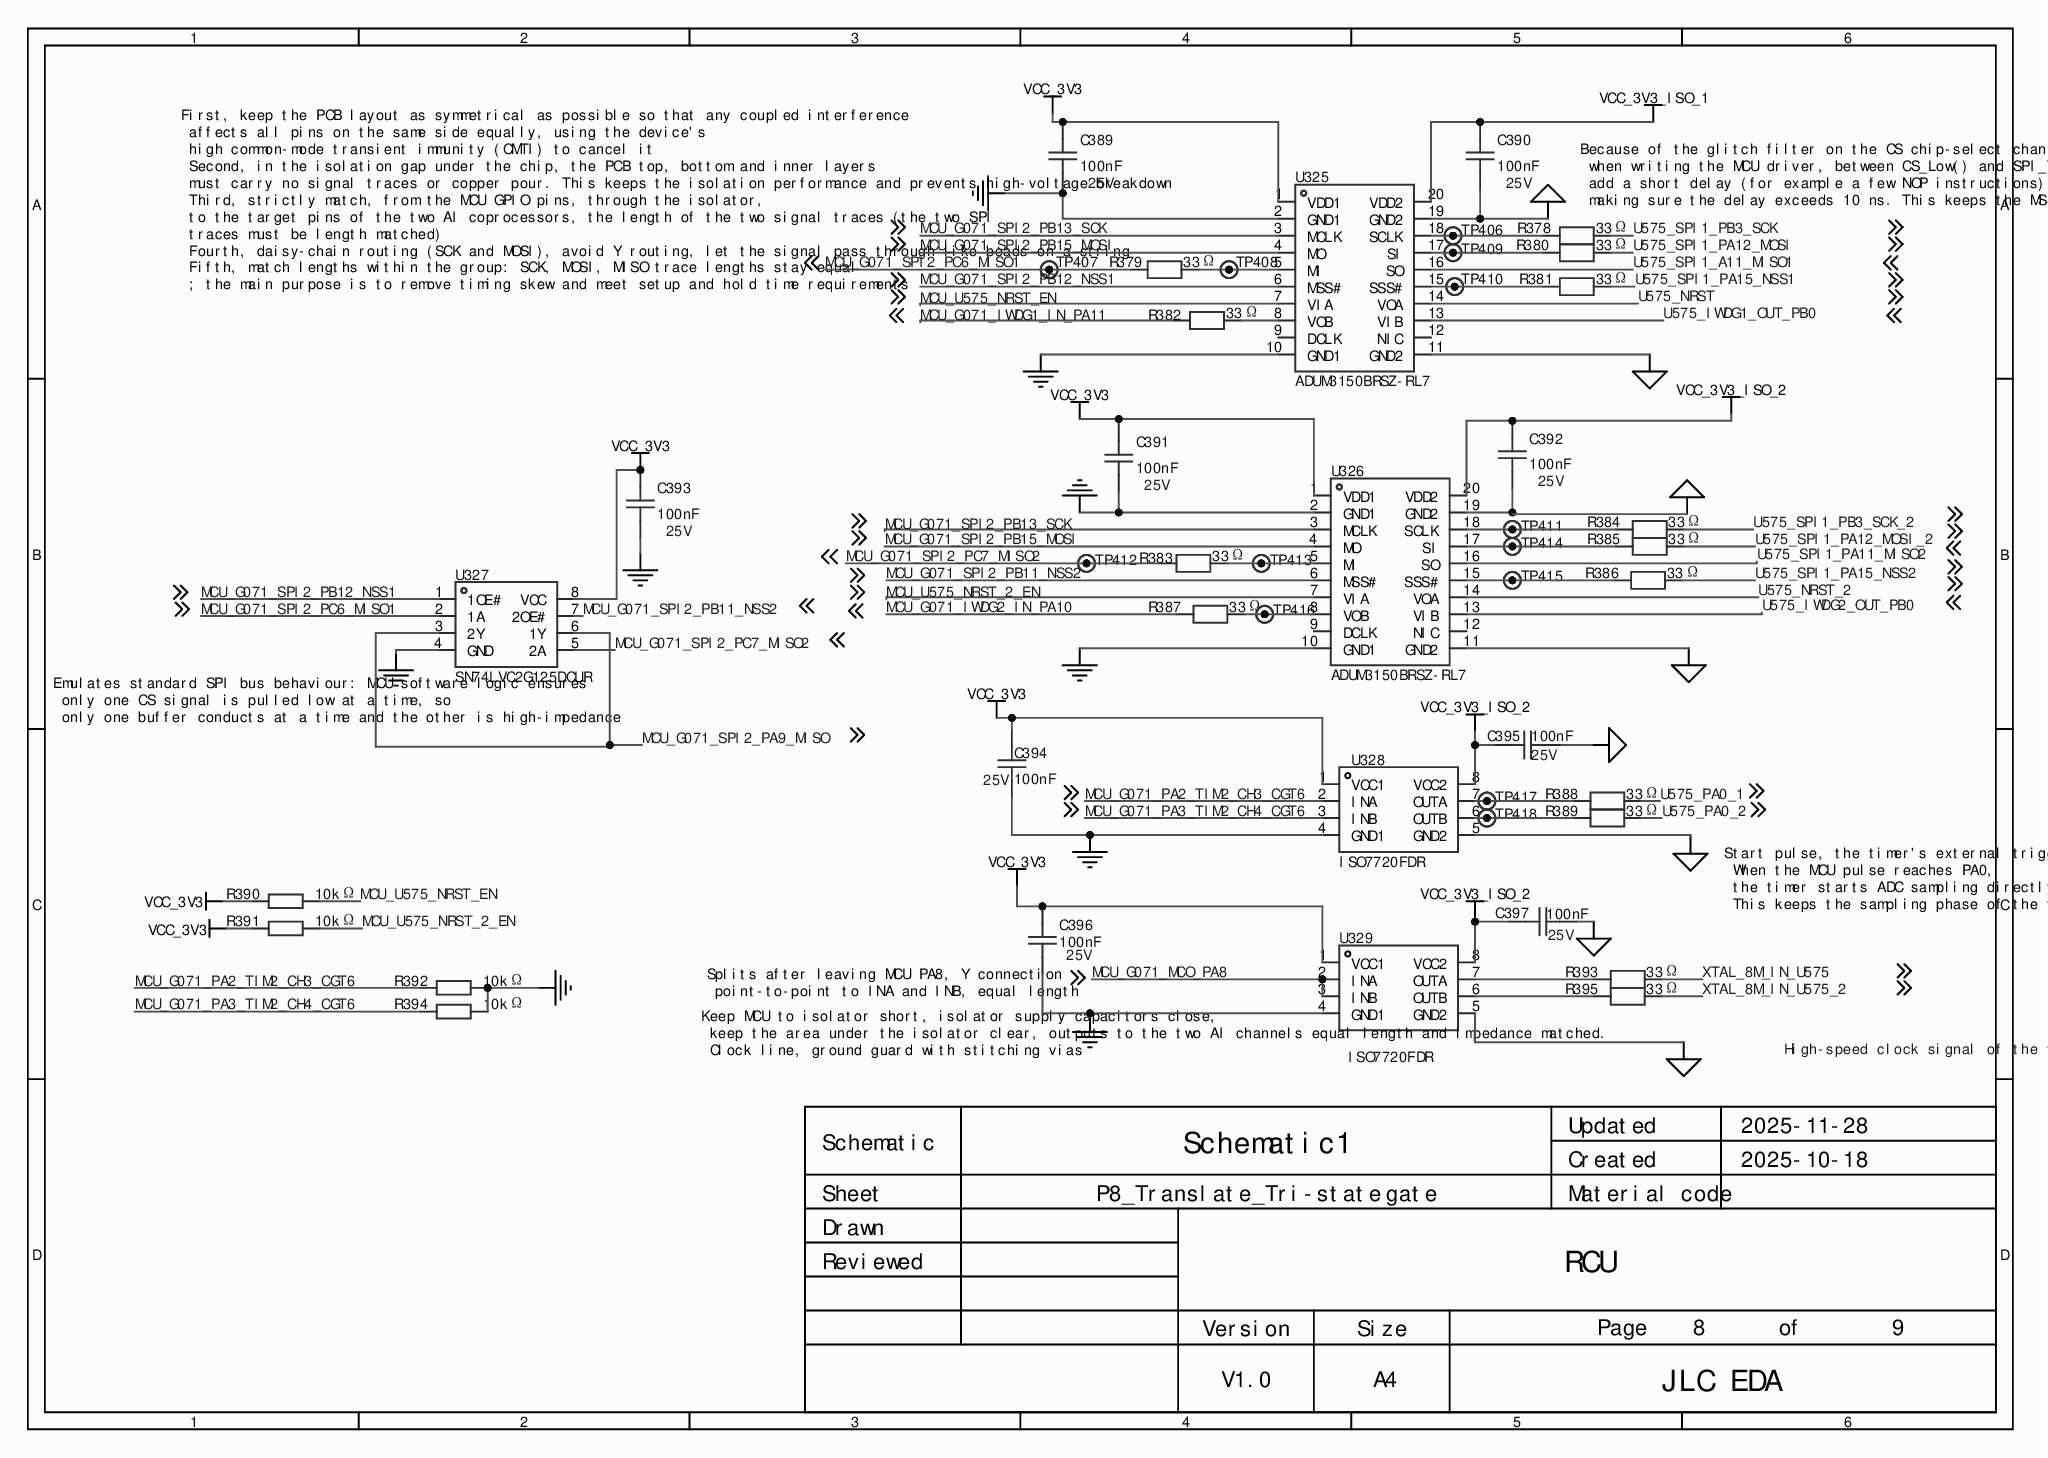
[diagram p0: MISC84429-10.SchDoc]
# Altium project MISC84429-12.PrjPcb (part 5 of 5)
## Sheet MISC84429-10.SchDoc (continued)
### Nets (continued)
U575_PA0_1: R388.1
U575_PA0_2: R389.1
U575_SPI1_A11_MISO1: U325.16(SO)
U575_SPI1_PA11_MISO2: U326.16(SO)
U575_SPI1_PA12_MOSI: R380.1
U575_SPI1_PA12_MOSI_2: R385.1
U575_SPI1_PA15_NSS1: R381.1
U575_SPI1_PA15_NSS2: R386.1
U575_SPI1_PB3_SCK: R378.1
U575_SPI1_PB3_SCK_2: R384.1
XTAL_8M_IN_U575: R393.1
XTAL_8M_IN_U575_2: R395.1
NetR378_2: R378.2 TP406.1 U325.18(SCLK)
NetR379_1: R379.1 TP408.1 U325.5(MI)
NetR380_2: R380.2 TP409.1 U325.17(SI)
NetR381_2: R381.2 TP410.1 U325.15(SSS#)
NetR382_1: R382.1 U325.8(VOB)
NetR383_1: R383.1 TP413.1 U326.5(MI)
NetR384_2: R384.2 TP411.1 U326.18(SCLK)
NetR385_2: R385.2 TP414.1 U326.17(SI)
NetR386_2: R386.2 TP415.1 U326.15(SSS#)
NetR387_1: R387.1 TP416.1 U326.8(VOB)
NetR388_2: R388.2 TP417.1 U328.7(OUTA)
NetR389_2: R389.2 TP418.1 U328.6(OUTB)
NetR393_2: R393.2 U329.7(OUTA)
NetR395_2: R395.2 U329.6(OUTB)

Not connected (* = marked no-connect by the designer): U325 9(DCLK)* 12(NIC)*; U326 9(DCLK)* 12(NIC)*

### Notes on the sheet
- First, keep the PCB layout as symmetrical as possible so that any coupled interference
  affects all pins on the same side equally, using the device's
  high common-mode transient immunity (CMTI) to cancel it
  Second, in the isolation gap under the chip, the PCB top, bottom and inner layers
  must carry no signal traces or copper pour. This keeps the isolation performance and prevents high-voltage breakdown
  Third, strictly match, from the MCU GPIO pins, through the isolator,
  to the target pins of the two AI coprocessors, the length of the two signal traces (the two SPI
  traces must be length matched)
  Fourth, daisy-chain routing (SCK and MOSI), avoid Y routing, let the signal pass through like beads on a string
  Fifth, match lengths within the group: SCK, MOSI, MISO trace lengths stay equal
  ; the main purpose is to remove timing skew and meet setup and hold time requirements
- Because of the glitch filter on the CS chip-select channel,
  when writing the MCU driver, between CS_Low() and SPI_Transmit()
  add a short delay (for example a few NOP instructions),
  making sure the delay exceeds 10 ns. This keeps the MSS setup time above 10ns
- Emulates standard SPI bus behaviour: MCU software logic ensures
  only one CS signal is pulled low at a time, so
  only one buffer conducts at a time and the other is high-impedance
- Start pulse, the timer's external trigger source.
  When the MCU pulse reaches PA0,
  the timer starts ADC sampling directly through the hardware link.
  This keeps the sampling phase of the two AI channels fully aligned
- Keep MCU to isolator short, isolator supply capacitors close,
  keep the area under the isolator clear, outputs to the two AI channels equal length and impedance matched.
  Clock line, ground guard with stitching vias
- Splits after leaving MCU PA8, Y connection
  point-to-point to INA and INB, equal length
- High-speed clock signal of the two AI coprocessors
- 1
- 2
- 3
- 4
- 5
- 6
- A
- B
- C
- Schematic
- Schematic1
- Created
- Updated
- 2025-11-28
- 2025-10-18
- D
- Reviewed
- Drawn
- Sheet
- P8_Translate_Tri-state gate
- Material code
- RCU
- Version
- Size
- Page
- 8
- of
- 9
- V1.0
- A4
- JLC EDA

### Library data of the parts
C389-C397 = GRM188R71E104KA01D: as C381-C384 on sheet MISC84429-8; Symbol: GRM188R71E104KA01D; Device: GRM188R71E104KA01D; LCSC Part Name: 100nF ±10% 25V; Supplier Part: C77050; Manufacturer Part: GRM188R71E104KA01D; Supplier Footprint: 0603; JLCPCB Part Class: Extended library; Datasheet: https://atta.szlcsc.com/upload/public/pdf/source/20170622/1498103881034.pdf; Supplier: LCSC; Convert to PCB: yes; Value: 100nF; Origin Footprint: C0603
R378-R389 R393 R395 = FRC0603F33R0TS: as R372 on sheet MISC84429-8; Symbol: FRC0603F33R0TS; Device: FRC0603F33R0TS; LCSC Part Name: 33Ω ±1% 100mW 厚膜电阻; Supplier Part: C2909394; Manufacturer Part: FRC0603F33R0TS; Supplier Footprint: 0603; JLCPCB Part Class: Extended library; Supplier: LCSC; Convert to PCB: yes; Type: Thick film resistor; Value: 33Ω; Operating Temperature: -55℃~+155℃; Origin Footprint: R0603
R390-R392 R394 = RC0603FR-0710KL: as R371 on sheet MISC84429-8; Symbol: RC0603FR-0710KL; Device: RC0603FR-0710KL; LCSC Part Name: 厚膜电阻 10kΩ ±1% 100mW; Supplier Part: C98220; Manufacturer Part: RC0603FR-0710KL; Supplier Footprint: 0603; JLCPCB Part Class: Extended library; Datasheet: https://atta.szlcsc.com/upload/public/pdf/source/20180927/C295883_E8D83085EA81BD7DE0B2B681138C15EE.pdf; Supplier: LCSC; Convert to PCB: yes; Type: Thick film resistor; Value: 10kΩ; Operating Temperature Range: -55℃~+155℃; Origin Footprint: R0603
TP406-TP418 = Test-Point: Add into BOM: yes; Symbol: Test-Point; Device: Test-Point; Convert to PCB: yes; Origin Footprint: Test-Point-0.5mm
U325 U326 = ADUM3150BRSZ-RL7: Manufacturer: ADI(亚德诺); Add into BOM: yes; Symbol: ADUM3150BRSZ-RL7; Device: ADUM3150BRSZ-RL7; LCSC Part Name: 用于SPI高速接口的3.75 kV专用隔离器（1/1辅助通道方向性）; Supplier Part: C660732; Manufacturer Part: ADUM3150BRSZ-RL7; Supplier Footprint: SSOP-20-208mil; JLCPCB Part Class: Extended library; Datasheet: https://atta.szlcsc.com/upload/public/pdf/source/20200914/C660732_9A8AE148C659C7DDC4EF09AB6B6BF7D1.pdf; Supplier: LCSC; Convert to PCB: yes; Origin Footprint: SSOP-20_L7.2-W5.3-P0.65-LS7.8-BL
U327 = SN74LVC2G125DCUR: Manufacturer: TI(德州仪器); Add into BOM: yes; output type: Tri-state; Voltage - Supply: 1.65V~5.5V; Number of Elements: 2; Current - Output Low(IOL): 32mA; Logic Family: 74LVC; Quiescent Current: 10uA; Propagation Delay: 4.3ns@3.3V,50pF; Symbol: SN74LVC2G125DCUR; Device: SN74LVC2G125DCUR; LCSC Part Name: 双路三态输出总线缓冲门; Supplier Part: C21404; Manufacturer Part: SN74LVC2G125DCUR; Supplier Footprint: VSSOP-8; JLCPCB Part Class: Extended library; Datasheet: https://www.ti.com/cn/lit/gpn/sn74lvc2g125; Supplier: LCSC; Convert to PCB: yes; Input type: -; Current - Output High(IOH): 32mA; Operating Temperature: -40℃~+85℃; Origin Footprint: VSON8_L2.0-W2.3-P0.50-LS3.1-BL
U328 U329 = ISO7720FDR: Manufacturer: TI(德州仪器); Add into BOM: yes; Number of Forward Channels: 2; Number of Reverse Channels: 0; Data Rate(Max): 100Mbps; Isolation Voltage(Vrms): 5000; CMTI(kV/us): 100kV/us; Voltage - Supply(VCCA): 2.25V~5.5V; Propagation Delay(tpd): 11ns; Symbol: ISO7720FDR; Device: ISO7720FDR; LCSC Part Name: ISO772x高速双通道增强型数字隔离器; Supplier Part: C2878308; Manufacturer Part: ISO7720FDR; Supplier Footprint: SOIC-8; JLCPCB Part Class: Extended library; Datasheet: https://www.ti.com/cn/lit/gpn/iso7721; Supplier: LCSC; Convert to PCB: yes; Default Output: -; Operating Temperature: -55℃~+125℃; Voltage - Supply(VCCB): 2.25V~5.5V; Origin Footprint: SOIC-8_L5.0-W4.0-P1.27-LS6.1-BL

## Sheet MISC84429-9.SchDoc
size 309 x 223 mm; Name: Sheet-Symbol; Symbol: Sheet-Symbol; Device: Sheet-Symbol
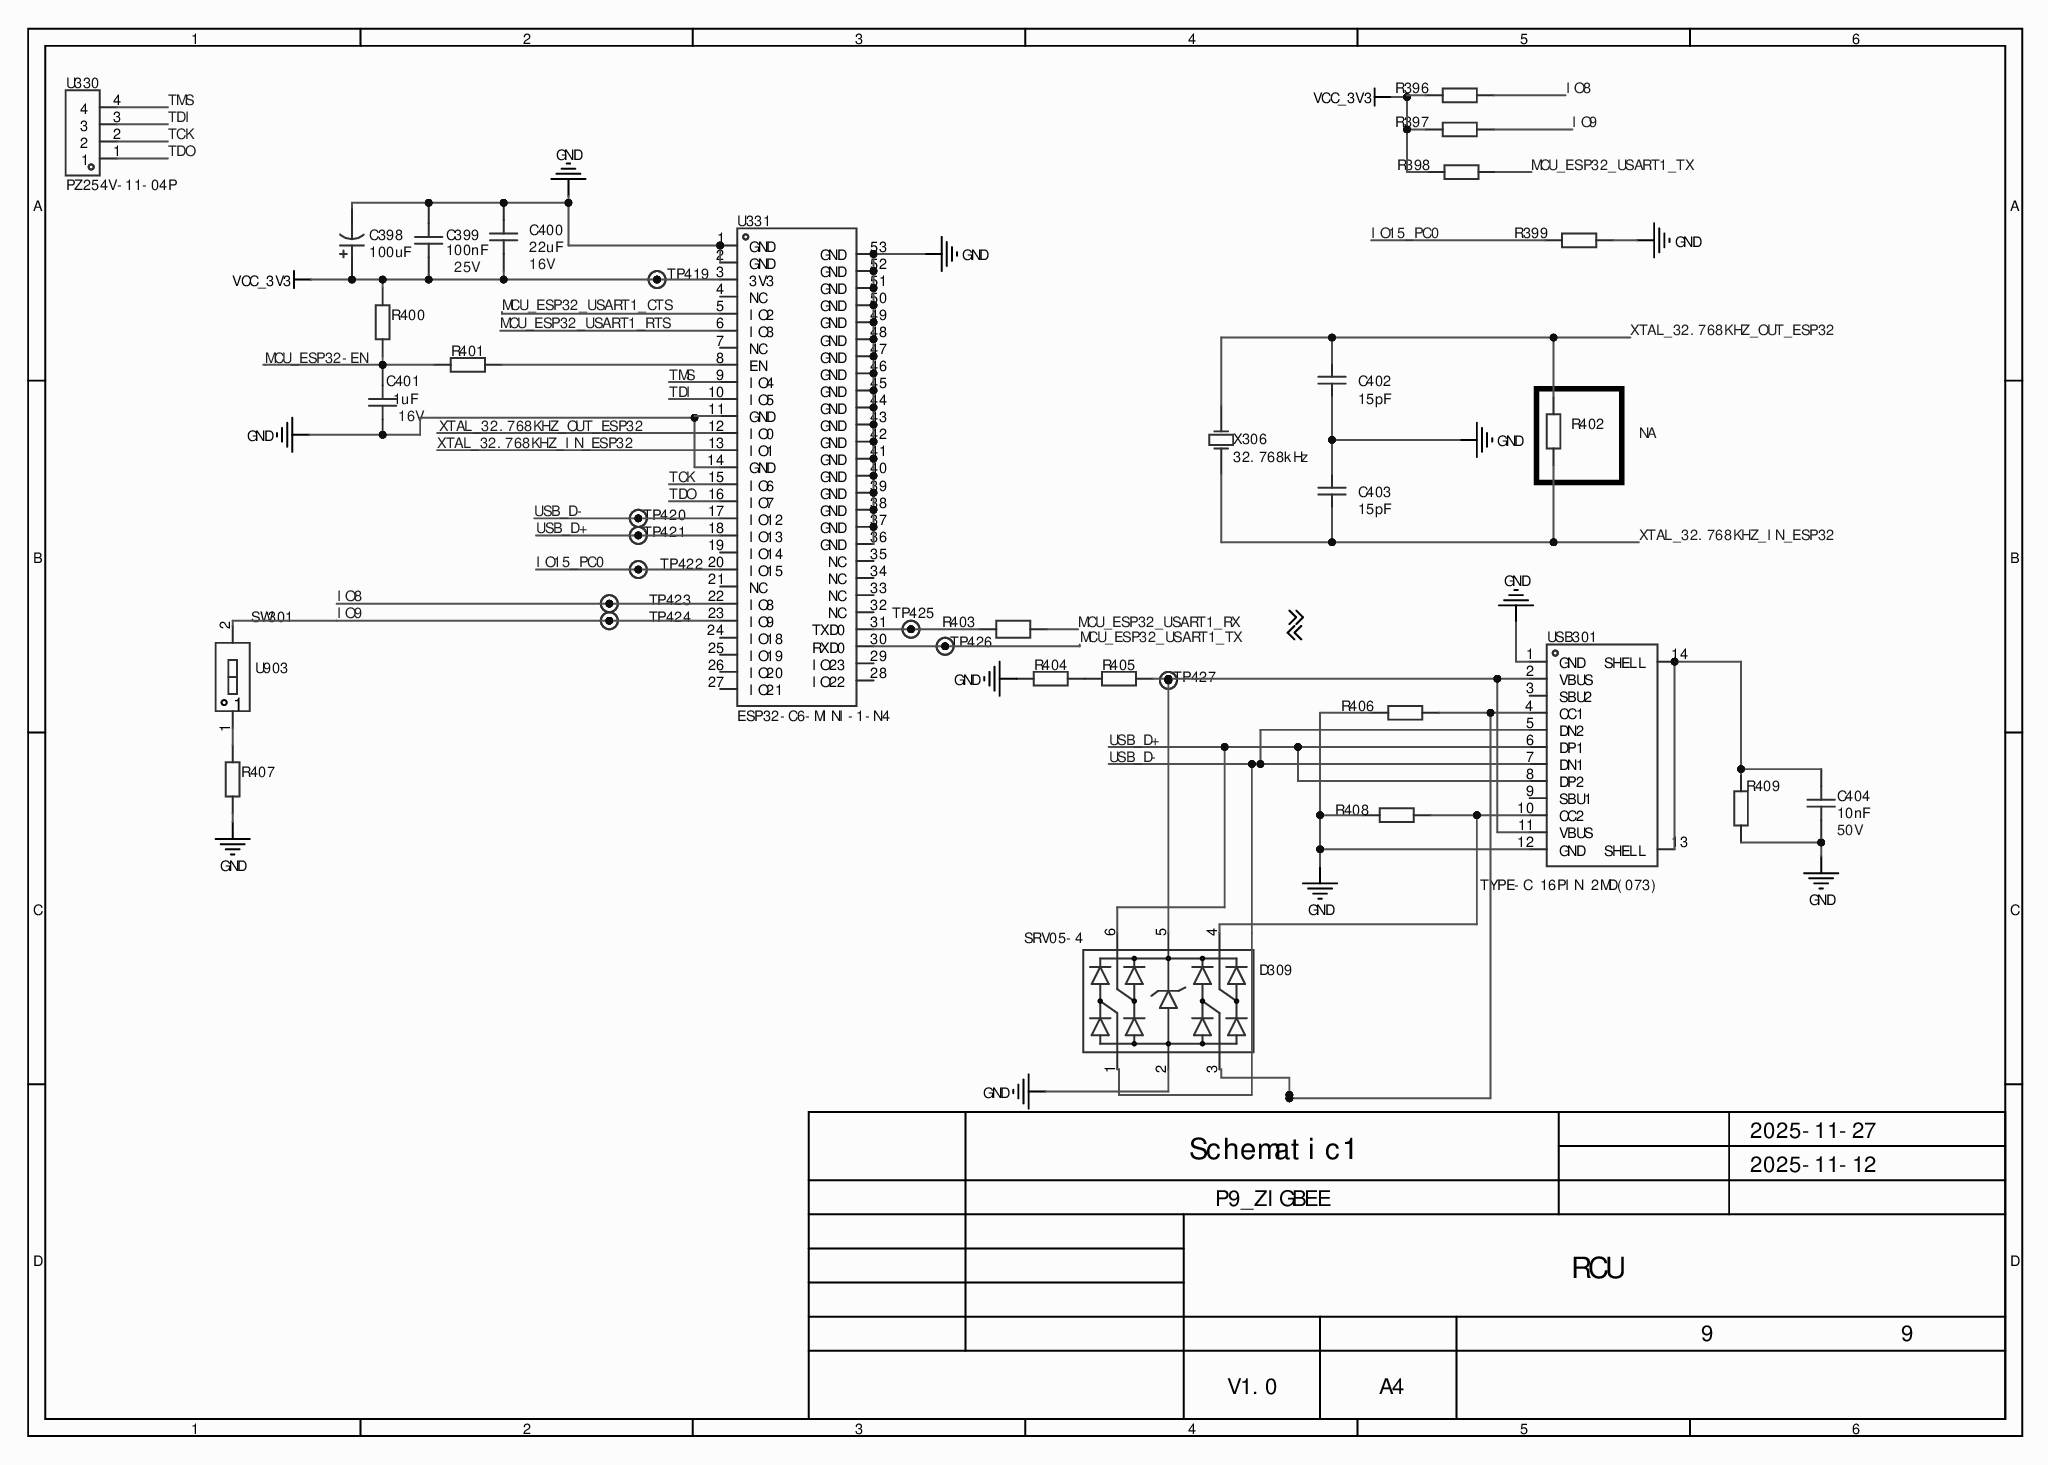
[diagram p1: MISC84429-9.SchDoc]

### Parts
C398  100uF  [CAP-SMD_BD6.3-L6.6-W6.6-LS7.2-FD]
C399  100nF  Voltage Rated: 25V  [C0603]
C400  22uF  Voltage Rating: 16V  [C0603]
C401  1uF  Voltage Rated: 16V  [C0603]
C402  15pF  [C0402]
C403  15pF  [C0402]
C404  10nF  Voltage Rating: 50V  [C0603]
D309  SRV05-4  [SOT-23-6_L2.9-W1.6-P0.95-LS2.8-BL]
R396  (no value)  [R0603]
R397  (no value)  [R0603]
R398  (no value)  [R0603]
R399  (no value)  [R0603]
R400  (no value)  [R0603]
R401  (no value)  [R0603]
R402  (no value)  [R0402]
R403  (no value)  [R0603]
R404  (no value)  [R0603]
R405  (no value)  [R0603]
R406  (no value)  [R0603]
R407  (no value)  [R0603]
R408  (no value)  [R0603]
R409  (no value)  [R0402]
SW301  U903  [SW-SMD_2P-L3.5-W6.1-P2.54-LS9.8]
TP419  (no value)  [Test-Point-0.5mm]
TP420  (no value)  [Test-Point-0.5mm]
TP421  (no value)  [Test-Point-0.5mm]
TP422  (no value)  [Test-Point-0.5mm]
TP423  (no value)  [Test-Point-0.5mm]
TP424  (no value)  [Test-Point-0.5mm]
TP425  (no value)  [Test-Point-0.5mm]
TP426  (no value)  [Test-Point-0.5mm]
TP427  (no value)  [Test-Point-0.5mm]
U330  PZ254V-11-04P  [HDR-TH_4P-P2.54-V-M]
U331  ESP32-C6-MINI-1-N4  [WIFIM-SMD_61P-L16.6-W13.2-P0.80-ESP32-C6-MINI-1-N4]
USB301  TYPE-C 16PIN 2MD(073)  [USB-C-SMD_TYPE-C-6PIN-2MD-073]
X306  32.768kHz  [OSC-TH_BD3.1-P0.8-D0.3]

### Nets
GND: C398.2 C399.1 C400.2 C401.1 C402.1 C403.2 C404.1 D309.2 R399.1 R404.2 R406.1 R407.1 R408.1 R409.1 U331.1(GND) U331.2(GND) U331.11(GND) U331.14(GND) U331.36(GND) U331.37(GND) U331.38(GND) U331.39(GND) U331.40(GND) U331.41(GND) U331.42(GND) U331.43(GND) U331.44(GND) U331.45(GND) U331.46(GND) U331.47(GND) U331.48(GND) U331.49(GND) U331.50(GND) U331.51(GND) U331.52(GND) U331.53(GND) USB301.1(GND) USB301.12(GND)
VCC_3V3: C398.1 C399.2 C400.1 R396.2 R397.2 R398.2 R400.2 TP419.1 U331.3(3V3)
IO8: R396.1 TP423.1 U331.22(IO8)
IO9: R397.1 SW301.2(PIN2) TP424.1 U331.23(IO9)
IO15_PC0: R399.2 TP422.1 U331.20(IO15)
MCU_ESP32-EN: C401.2 R400.1 R401.1
MCU_ESP32_USART1_CTS: U331.5(IO2)
MCU_ESP32_USART1_RTS: U331.6(IO3)
MCU_ESP32_USART1_RX: R403.1
MCU_ESP32_USART1_TX: R398.1 TP426.1 U331.30(RXD0)
TCK: U330.2 U331.15(IO6)
TDI: U330.3 U331.10(IO5)
TDO: U330.1 U331.16(IO7)
TMS: U330.4 U331.9(IO4)
USB_D+: D309.6 TP421.1 U331.18(IO13) USB301.6(DP1) USB301.8(DP2)
USB_D-: D309.1 TP420.1 U331.17(IO12) USB301.5(DN2) USB301.7(DN1)
XTAL_32.768KHZ_IN_ESP32: C403.1 R402.1 U331.13(IO1) X306.2(OSC2)
XTAL_32.768KHZ_OUT_ESP32: C402.2 R402.2 U331.12(IO0) X306.1(OSC1)
NetC404_2: C404.2 R409.2 USB301.13(SHELL) USB301.14(SHELL)
NetD309_3: D309.3 R406.2 USB301.4(CC1)
NetD309_4: D309.4 R408.2 USB301.10(CC2)
NetD309_5: D309.5 R405.2 TP427.1 USB301.2(VBUS) USB301.11(VBUS)
NetR401_2: R401.2 U331.8(EN)
NetR403_2: R403.2 TP425.1 U331.31(TXD0)
NetR404_1: R404.1 R405.1
NetR407_2: R407.2 SW301.1(PIN1)

Not connected (* = marked no-connect by the designer): U331 4(NC)* 7(NC)* 19(IO14)* 21(NC)* 24(IO18)* 25(IO19)* 26(IO20)* 27(IO21)* 28(IO22)* 29(IO23)* 32(NC)* 33(NC)* 34(NC)* 35(NC)*; USB301 3(SBU2)* 9(SBU1)*

### Notes on the sheet
- NA
- 1
- 2
- 3
- 4
- 5
- 6
- A
- B
- C
- Schematic1
- 2025-11-27
- 2025-11-12
- D
- P9_ZIGBEE
- RCU
- 9
- V1.0
- A4

### Library data of the parts
C398 = 100uF: Symbol: RVT100UF16V67RV0016; Add into BOM: yes; Voltage Rating: 16V; Ripple Current: 93mA@120Hz; Device: 100uF; Supplier Part: C2887276; Manufacturer Part: RVT100UF16V67RV0016; Supplier Footprint: SMD,D6.3xL5.4mm; Datasheet: https://atta.szlcsc.com/upload/public/pdf/source/20240521/3810EB5B434F72326C196D6A9426C70A.pdf; Supplier: LCSC; Convert to PCB: yes; Value: 100uF; Equivalent Series Resistance(ESR): -; Diameter: 6.3mm; Height - Seated (Max): 5.4mm; Origin Footprint: CAP-SMD_BD6.3-L6.6-W6.6-LS7.2-FD; Design Item ID: RVT100UF16V67RV0016
C399 = 100nF: Symbol: GRM188R71E104KA01D; Add into BOM: yes; Temperature Coefficient: X7R; Device: 100nF; Supplier Part: C77050; Manufacturer Part: GRM188R71E104KA01D; Supplier Footprint: 0603; Datasheet: https://atta.szlcsc.com/upload/public/pdf/source/20170622/1498103881034.pdf; Supplier: LCSC; Convert to PCB: yes; Value: 100nF; Origin Footprint: C0603; Design Item ID: GRM188R71E104KA01D
C400 = 22uF: Symbol: GRM188R61C226ME01D; Add into BOM: yes; Temperature Coefficient: X5R; Device: 22uF; Supplier Part: C5116073; Manufacturer Part: GRM188R61C226ME01D; Supplier Footprint: 0603; Datasheet: https://item.szlcsc.com/datasheet/GRM188R61C226ME01D/5691201.html; Supplier: LCSC; Convert to PCB: yes; Value: 22uF; Origin Footprint: C0603; Design Item ID: GRM188R61C226ME01D
C401 = 1uF: Symbol: GCM188R71C105KA64D; Add into BOM: yes; Temperature Coefficient: X7R; Device: 1uF; Supplier Part: C161212; Manufacturer Part: GCM188R71C105KA64D; Supplier Footprint: 0603; Datasheet: https://atta.szlcsc.com/upload/public/pdf/source/20181221/C161212_C96DD77354D5551432B3B7779E4D1948.pdf; Supplier: LCSC; Convert to PCB: yes; Value: 1uF; Origin Footprint: C0603; Design Item ID: GCM188R71C105KA64D
C402 C403 = 15pF: Symbol: GJM1555C1H150FB01D; Add into BOM: yes; Voltage Rated: 50V; Temperature Coefficient: C0G; Device: 15pF; Supplier Part: C441742; Manufacturer Part: GJM1555C1H150FB01D; Supplier Footprint: 0402; Datasheet: https://atta.szlcsc.com/upload/public/pdf/source/20200305/C490387_23319AE8C154DEB24C505E6C82A8106A.pdf; Supplier: LCSC; Convert to PCB: yes; Value: 15pF; Origin Footprint: C0402; Design Item ID: GJM1555C1H150FB01D
C404 = 10nF: Symbol: GCM188R71H103KA37D; Add into BOM: yes; Temperature Coefficient: X7R; Device: 10nF; Supplier Part: C85863; Manufacturer Part: GCM188R71H103KA37D; Supplier Footprint: 0603; Datasheet: https://item.szlcsc.com/datasheet/GCM188R71H103KA37D/87039.html; Supplier: LCSC; Convert to PCB: yes; Value: 10nF; Origin Footprint: C0603; Design Item ID: GCM188R71H103KA37D
D309 = SRV05-4: Symbol: SRV05-4_C558418; Add into BOM: yes; Reverse Stand-Off Voltage (Vrwm): 5V; Clamping Voltage: 20V; Peak Pulse Current (Ipp): 3A; Peak Pulse Power Dissipation (Ppp): 60W; Voltage - Breakdown: 6V; Reverse Leakage Current (Ir): 500nA; Type: ESD; Device: SRV05-4; Supplier Part: C558418; Manufacturer Part: SRV05-4; Supplier Footprint: SOT-23-6; Datasheet: https://item.szlcsc.com/datasheet/SRV05-4/581825.html; Supplier: LCSC; Convert to PCB: yes; Origin Footprint: SOT-23-6_L2.9-W1.6-P0.95-LS2.8-BL; Design Item ID: SRV05-4_C558418
R396-R399 R407 = RC0603FR-074K7L: Add into BOM: yes; Power(Watts): 100mW; Voltage-Supply(Max): 75V; Symbol: RC0603FR-074K7L; Device: RC0603FR-074K7L; Supplier Part: C99782; Manufacturer Part: RC0603FR-074K7L; Supplier Footprint: 0603; Datasheet: https://atta.szlcsc.com/upload/public/pdf/source/20250610/89E4D743C004A82A45145C7A2CC3A578.pdf; Supplier: LCSC; Convert to PCB: yes; Origin Footprint: R0603; Design Item ID: RC0603FR-074K7L
R400 R404 R405 = RC0603FR-0710KL: Add into BOM: yes; Power(Watts): 100mW; Overload Voltage (Max): 75V; Symbol: RC0603FR-0710KL; Device: RC0603FR-0710KL; Supplier Part: C98220; Manufacturer Part: RC0603FR-0710KL; Supplier Footprint: 0603; Datasheet: https://atta.szlcsc.com/upload/public/pdf/source/20180927/C295883_E8D83085EA81BD7DE0B2B681138C15EE.pdf; Supplier: LCSC; Convert to PCB: yes; Origin Footprint: R0603; Design Item ID: RC0603FR-0710KL
R401 = RC0603FR-070RL: Add into BOM: yes; Power(Watts): 100mW; Voltage-Supply(Max): 75V; Symbol: RC0603FR-070RL; Device: RC0603FR-070RL; Supplier Part: C100044; Manufacturer Part: RC0603FR-070RL; Supplier Footprint: 0603; Datasheet: https://item.szlcsc.com/datasheet/RC0603FR-070RL/101258.html; Supplier: LCSC; Convert to PCB: yes; Temperature Coefficient: -; Origin Footprint: R0603; Design Item ID: RC0603FR-070RL
R402 = 0402WGF1002TCE: Add into BOM: yes; Power(Watts): 62.5mW; Overload Voltage (Max): 50V; Symbol: 0402WGF1002TCE; Device: 0402WGF1002TCE; Supplier Part: C25744; Manufacturer Part: 0402WGF1002TCE; Supplier Footprint: 0402; Datasheet: https://atta.szlcsc.com/upload/public/pdf/source/20200306/C422600_1E6D84923E4A46A82E41ADD87F860B5C.pdf; Supplier: LCSC; Convert to PCB: yes; Origin Footprint: R0402; Design Item ID: 0402WGF1002TCE
R403 = FRC0603F33R0TS: Add into BOM: yes; Power(Watts): 100mW; Voltage-Supply(Max): 75V; Symbol: FRC0603F33R0TS; Device: FRC0603F33R0TS; Supplier Part: C2909394; Manufacturer Part: FRC0603F33R0TS; Supplier Footprint: 0603; Supplier: LCSC; Convert to PCB: yes; Origin Footprint: R0603; Design Item ID: FRC0603F33R0TS
R406 R408 = RC0603FR-075K1L: Add into BOM: yes; Power(Watts): 100mW; Voltage-Supply(Max): 75V; Symbol: RC0603FR-075K1L; Device: RC0603FR-075K1L; Supplier Part: C105580; Manufacturer Part: RC0603FR-075K1L; Supplier Footprint: 0603; Datasheet: https://atta.szlcsc.com/upload/public/pdf/source/20180316/70C0E2BDAE7FCC62C531A5A58D202EE1.pdf; Supplier: LCSC; Convert to PCB: yes; Origin Footprint: R0603; Design Item ID: RC0603FR-075K1L
R409 = 0402WGF1004TCE: Add into BOM: yes; Power(Watts): 62.5mW; Overload Voltage (Max): 50V; Symbol: 0402WGF1004TCE; Device: 0402WGF1004TCE; Supplier Part: C26083; Manufacturer Part: 0402WGF1004TCE; Supplier Footprint: 0402; Datasheet: https://atta.szlcsc.com/upload/public/pdf/source/20200306/C422600_1E6D84923E4A46A82E41ADD87F860B5C.pdf; Supplier: LCSC; Convert to PCB: yes; Origin Footprint: R0402; Design Item ID: 0402WGF1004TCE
SW301 = U903: Symbol: DSIC01LS-P; Add into BOM: yes; Current Rating: 25mA; Voltage Rating: 24V; Device: U903; Supplier Part: C600988; Manufacturer Part: U903; Supplier Footprint: SMD,6.2x3.5mm; Datasheet: https://item.szlcsc.com/datasheet/DSIC01LS-P/631008.html; Supplier: LCSC; Convert to PCB: yes; Lead Pitch: -; Origin Footprint: SW-SMD_2P-L3.5-W6.1-P2.54-LS9.8; Design Item ID: DSIC01LS-P
TP419-TP427 = Test-Point: Add into BOM: yes; Symbol: Test-Point; Device: Test-Point; Convert to PCB: yes; Origin Footprint: Test-Point-0.5mm; Design Item ID: Test-Point
U330 = PZ254V-11-04P: Add into BOM: yes; Pin Structure: 1x4P; Pitch: 2.54mm; Current Rating: 3A; Voltage Rating (Max): 250V; Symbol: PZ254V-11-04P; Device: PZ254V-11-04P; Supplier Part: C2691448; Manufacturer Part: PZ254V-11-04P; Datasheet: https://item.szlcsc.com/datasheet/PZ254V-11-04P/2801085.html; Supplier: LCSC; Convert to PCB: yes; Row Spacing: -; Number of Pins: 4P; Length of Mating Pin: 6mm; Insulation Height: 2.5mm; Length of End Connection Pin: 3mm; Contact Material: -; Origin Footprint: HDR-TH_4P-P2.54-V-M; Design Item ID: PZ254V-11-04P
U331 = ESP32-C6-MINI-1-N4: Add into BOM: yes; Symbol: ESP32-C6-MINI-1-N4; Device: ESP32-C6-MINI-1-N4; LCSC Part Name: ESP32-C6-MINI-1-N4; Supplier Part: C5736265; Manufacturer Part: ESP32-C6-MINI-1-N4; Supplier Footprint: SMD-53P; Datasheet: https://item.szlcsc.com/datasheet/ESP32-C6-MINI-1-N4/6661848.html; Supplier: LCSC; Convert to PCB: yes; Origin Footprint: WIFIM-SMD_61P-L16.6-W13.2-P0.80-ESP32-C6-MINI-1-N4; Design Item ID: ESP32-C6-MINI-1-N4
USB301 = TYPE-C 16PIN 2MD(073): Add into BOM: yes; Number of Contacts: 16P; Number of Ports: 1; Current Rating-Power: 3A; Voltage Rating: 5V; Symbol: TYPE-C 16PIN 2MD(073); Device: TYPE-C 16PIN 2MD(073); Supplier Part: C2765186; Manufacturer Part: TYPE-C 16PIN 2MD(073); Supplier Footprint: SMD; Datasheet: https://item.szlcsc.com/datasheet/TYPE-C%252016PIN%25202MD(073)/2901843.html; Supplier: LCSC; Convert to PCB: yes; Connector Type: Type-C; Protocol Standard: -; Supplementary Features: -; Center Height: -; Length: -; Origin Footprint: USB-C-SMD_TYPE-C-6PIN-2MD-073; Design Item ID: TYPE-C 16PIN 2MD(073)
X306 = 32.768kHz: Symbol: X308032768KGB2SC; Add into BOM: yes; Load Capacitance: 12.5pF; Device: 32.768kHz; Supplier Part: C52082; Manufacturer Part: X308032768KGB2SC; Supplier Footprint: DT-38; Datasheet: https://item.szlcsc.com/datasheet/X308032768KGB2SC/53096.html; Supplier: LCSC; Convert to PCB: yes; Value: 32.768kHz; Origin Footprint: OSC-TH_BD3.1-P0.8-D0.3; Design Item ID: X308032768KGB2SC

## Nets that join several sheets
GND: MISC84429-4 (26 pins), MISC84429-3 (11 pins), MISC84429-5 (11 pins), MISC84429-6 (18 pins), MISC84429-10 (14 pins), MISC84429-9 (38 pins)
PGND: MISC84429-7 (20 pins), MISC84429-4 (19 pins), MISC84429-8 (23 pins), MISC84429-10 (10 pins)
VCC_3V3: MISC84429-4 (5 pins), MISC84429-5 (11 pins), MISC84429-6 (15 pins), MISC84429-10 (12 pins), MISC84429-9 (9 pins)
VCC_3V3_ISO_1: MISC84429-7 (17 pins), MISC84429-4 (C324.1 C325.2 TP316.1 U308.14), MISC84429-10 (C390.1 U325.20)
VCC_3V3_ISO_2: MISC84429-4 (C330.1 C331.2 TP318.1 U309.14), MISC84429-8 (17 pins), MISC84429-10 (6 pins)
VCC_5V: MISC84429-4 (8 pins), MISC84429-3 (7 pins)
VCC_6V5: MISC84429-3 (C421.1 C422.2 L311.2 TP428.1), MISC84429-5 (C415.2 R416.1 U335.4)
220V_N_OUT: MISC84429-3 (8 pins), MISC84429-5 (35 pins)
220V_RELAY_OUT: MISC84429-3 (U303.5 U303.6), MISC84429-5 (U315.1)
220V_TRANSFORMER_OUT: MISC84429-3 (U302.1), MISC84429-5 (L308.1 U315.3)
MCU_CBT6_PA0_ZCR: MISC84429-5 (U339.14), MISC84429-6 (TP353.1 U316.11)
MCU_CBT6_PA1_SYN: MISC84429-5 (C339.1 R331.2 U339.11), MISC84429-6 (TP355.1 U316.12)
MCU_CBT6_PA4_INT1: MISC84429-5 (U339.13), MISC84429-6 (TP365.1 U316.15)
MCU_CBT6_PB1_IS3115_EN1: MISC84429-4 (C327.2 R324.1 TP314.1 U308.1), MISC84429-6 (U316.20)
MCU_CBT6_PB2_IS3115_EN2: MISC84429-4 (C326.2 R325.1 TP317.1 U309.1), MISC84429-6 (U316.21)
MCU_ESP32_USART1_CTS: MISC84429-6 (TP348.1 U316.43), MISC84429-9 (U331.5)
MCU_ESP32_USART1_RTS: MISC84429-6 (TP349.1 U316.42), MISC84429-9 (U331.6)
MCU_ESP32_USART1_RX: MISC84429-6 (TP344.1 U316.46), MISC84429-9 (R403.1)
MCU_ESP32_USART1_TX: MISC84429-6 (R346.1 TP347.1), MISC84429-9 (R398.1 TP426.1 U331.30)
MCU_G071_IWDG1_IN_PA11: MISC84429-6 (TP362.1 U316.33), MISC84429-10 (R382.2)
MCU_G071_IWDG2_IN_PA10: MISC84429-6 (TP369.1 U316.32), MISC84429-10 (R387.2)
MCU_G071_MCO_PA8: MISC84429-6 (R351.1), MISC84429-10 (U329.2 U329.3)
MCU_G071_PA2_TIM2_CH3_CGT6: MISC84429-6 (TP357.1 U316.13), MISC84429-10 (R392.1 U328.2)
MCU_G071_PA3_TIM2_CH4_CGT6: MISC84429-6 (TP358.1 U316.14), MISC84429-10 (R394.1 U328.3)
MCU_G071_SPI2_PA9_MISO: MISC84429-6 (U316.29), MISC84429-10 (U327.3 U327.6)
MCU_G071_SPI2_PB11_NSS2: MISC84429-6 (TP371.1 U316.23), MISC84429-10 (U326.6 U327.7)
MCU_G071_SPI2_PB12_NSS1: MISC84429-6 (TP374.1 U316.24), MISC84429-10 (U325.6 U327.1)
MCU_G071_SPI2_PB13_SCK: MISC84429-6 (R353.1 TP376.1), MISC84429-10 (U325.3 U326.3)
MCU_G071_SPI2_PB15_MOSI: MISC84429-6 (R352.1 TP373.1), MISC84429-10 (U325.4 U326.4)
MCU_PA5_SPI1_SCK: MISC84429-5 (C338.1 R329.2 U337.3), MISC84429-6 (R348.2 TP361.1)
MCU_PA6_SPI1_MISO: MISC84429-5 (C336.1 R326.2 U337.6), MISC84429-6 (TP364.1 U316.17)
MCU_PA7_SPI1_MOSI: MISC84429-5 (C337.1 R327.2 U337.4), MISC84429-6 (R349.2 TP363.1)
MCU_PB0_SPI1_CS: MISC84429-5 (C341.1 R332.2 U337.5), MISC84429-6 (R350.2 TP367.1)
MCU_RELAY_CTL_PD3: MISC84429-3 (R306.1), MISC84429-6 (TP350.1 U316.41)
MCU_STPM32_EN_PD2: MISC84429-5 (U339.12), MISC84429-6 (TP352.1 U316.40)
MCU_U575_NRST_2_EN: MISC84429-6 (TP356.1 U316.38), MISC84429-10 (R391.2 U326.7)
MCU_U575_NRST_EN: MISC84429-6 (TP354.1 U316.39), MISC84429-10 (R390.2 U325.7)
U575_IWDG1_OUT_PB0: MISC84429-7 (R361.2 TP381.1), MISC84429-10 (U325.13)
U575_IWDG2_OUT_PB0: MISC84429-8 (R372.2 TP394.1), MISC84429-10 (U326.13)
U575_NRST: MISC84429-7 (8 pins), MISC84429-10 (U325.14)
U575_NRST_2: MISC84429-8 (8 pins), MISC84429-10 (U326.14)
U575_PA0_1: MISC84429-7 (TP379.1 U319.10), MISC84429-10 (R388.1)
U575_PA0_2: MISC84429-8 (TP392.1 U322.10), MISC84429-10 (R389.1)
U575_SPI1_A11_MISO1: MISC84429-7 (R364.1 TP386.1), MISC84429-10 (U325.16)
U575_SPI1_PA11_MISO2: MISC84429-8 (R373.1 TP399.1), MISC84429-10 (U326.16)
U575_SPI1_PA12_MOSI: MISC84429-7 (TP385.1 U319.33), MISC84429-10 (R380.1)
U575_SPI1_PA12_MOSI_2: MISC84429-8 (TP398.1 U322.33), MISC84429-10 (R385.1)
U575_SPI1_PA15_NSS1: MISC84429-7 (TP389.1 U319.38), MISC84429-10 (R381.1)
U575_SPI1_PA15_NSS2: MISC84429-8 (TP402.1 U322.38), MISC84429-10 (R386.1)
U575_SPI1_PB3_SCK: MISC84429-7 (TP383.1 U319.39), MISC84429-10 (R378.1)
U575_SPI1_PB3_SCK_2: MISC84429-8 (TP396.1 U322.39), MISC84429-10 (R384.1)
XTAL_8M_IN_U575: MISC84429-7 (U319.5), MISC84429-10 (R393.1)
XTAL_8M_IN_U575_2: MISC84429-8 (U322.5), MISC84429-10 (R395.1)